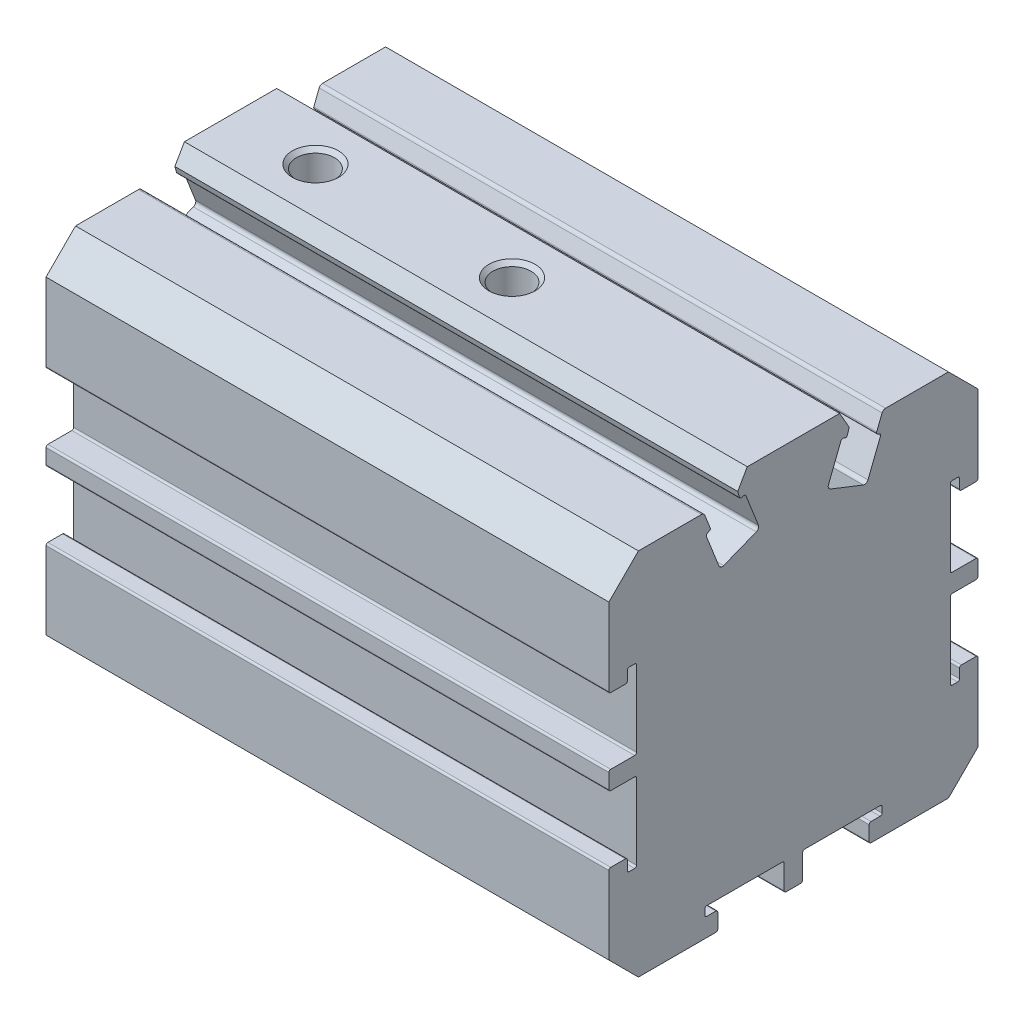
from build123d import *

# Parameters (mm, degrees)
BOSS_EXTRUDE1_DEPTH  = 61
LPATTERN1_COUNT      = 2
LPATTERN1_PITCH      = 28
LPATTERN1_COUNT_DIR2 = 2
LPATTERN1_PITCH_DIR2 = 28
BOSS_EXTRUDE2_START  = 1.2
SKETCH8_R            = 1
BOSS_EXTRUDE2_DEPTH  = 1.2


with BuildPart() as part:
    # Sketch1 → Boss-Extrude1 (new body)
    with BuildSketch(Plane(origin=(0, 0, 0), x_dir=(0, 0, -1), z_dir=(1, 0, 0))):
        with BuildLine():
            Line((-20, 16.8), (-20, 8.4))
            ThreePointArc((-20, 8.4), (-19.941421356, 8.258578644), (-19.8, 8.2))
            Line((-19.8, 8.2), (-18.2, 8.2))
            ThreePointArc((-18.2, 8.2), (-18.058578644, 8.258578644), (-18, 8.4))
            Line((-18, 8.4), (-18, 9.4))
            ThreePointArc((-18, 9.4), (-17.941421356, 9.541421356), (-17.8, 9.6))
            Line((-17.8, 9.6), (-17.2, 9.6))
            ThreePointArc((-17.2, 9.6), (-17.058578644, 9.541421356), (-17, 9.4))
            Line((-17, 9.4), (-17, 1.2))
            ThreePointArc((-17, 1.2), (-17.058578644, 1.058578644), (-17.2, 1))
            Line((-17.2, 1), (-19.8, 1))
            ThreePointArc((-19.8, 1), (-19.941421356, 0.941421356), (-20, 0.8))
            Line((-20, 0.8), (-20, -0.8))
            ThreePointArc((-20, -0.8), (-19.941421356, -0.941421356), (-19.8, -1))
            Line((-19.8, -1), (-17.2, -1))
            ThreePointArc((-17.2, -1), (-17.058578644, -1.058578644), (-17, -1.2))
            Line((-17, -1.2), (-17, -9.4))
            ThreePointArc((-17, -9.4), (-17.058578644, -9.541421356), (-17.2, -9.6))
            Line((-17.2, -9.6), (-17.8, -9.6))
            ThreePointArc((-17.8, -9.6), (-17.941421356, -9.541421356), (-18, -9.4))
            Line((-18, -9.4), (-18, -8.4))
            ThreePointArc((-18, -8.4), (-18.058578644, -8.258578644), (-18.2, -8.2))
            Line((-18.2, -8.2), (-19.8, -8.2))
            ThreePointArc((-19.8, -8.2), (-19.941421356, -8.258578644), (-20, -8.4))
            Line((-20, -8.4), (-20, -16.8))
            Line((-20, -16.8), (-16.8, -20))
            Line((-16.8, -20), (-8.4, -20))
            ThreePointArc((-8.4, -20), (-8.258578644, -19.941421356), (-8.2, -19.8))
            Line((-8.2, -19.8), (-8.2, -18.2))
            ThreePointArc((-8.2, -18.2), (-8.258578644, -18.058578644), (-8.4, -18))
            Line((-8.4, -18), (-9.4, -18))
            ThreePointArc((-9.4, -18), (-9.541421356, -17.941421356), (-9.6, -17.8))
            Line((-9.6, -17.8), (-9.6, -17.2))
            ThreePointArc((-9.6, -17.2), (-9.541421356, -17.058578644), (-9.4, -17))
            Line((-9.4, -17), (-1.2, -17))
            ThreePointArc((-1.2, -17), (-1.058578644, -17.058578644), (-1, -17.2))
            Line((-1, -17.2), (-1, -19.8))
            ThreePointArc((-1, -19.8), (-0.941421356, -19.941421356), (-0.8, -20))
            Line((-0.8, -20), (0.8, -20))
            ThreePointArc((0.8, -20), (0.941421356, -19.941421356), (1, -19.8))
            Line((1, -19.8), (1, -17.2))
            ThreePointArc((1, -17.2), (1.058578644, -17.058578644), (1.2, -17))
            Line((1.2, -17), (9.4, -17))
            ThreePointArc((9.4, -17), (9.541421356, -17.058578644), (9.6, -17.2))
            Line((9.6, -17.2), (9.6, -17.8))
            ThreePointArc((9.6, -17.8), (9.541421356, -17.941421356), (9.4, -18))
            Line((9.4, -18), (8.4, -18))
            ThreePointArc((8.4, -18), (8.258578644, -18.058578644), (8.2, -18.2))
            Line((8.2, -18.2), (8.2, -19.8))
            ThreePointArc((8.2, -19.8), (8.258578644, -19.941421356), (8.4, -20))
            Line((8.4, -20), (16.8, -20))
            Line((16.8, -20), (20, -16.8))
            Line((20, -16.8), (20, -8.4))
            ThreePointArc((20, -8.4), (19.941421356, -8.258578644), (19.8, -8.2))
            Line((19.8, -8.2), (18.2, -8.2))
            ThreePointArc((18.2, -8.2), (18.058578644, -8.258578644), (18, -8.4))
            Line((18, -8.4), (18, -9.4))
            ThreePointArc((18, -9.4), (17.941421356, -9.541421356), (17.8, -9.6))
            Line((17.8, -9.6), (17.2, -9.6))
            ThreePointArc((17.2, -9.6), (17.058578644, -9.541421356), (17, -9.4))
            Line((17, -9.4), (17, -1.2))
            ThreePointArc((17, -1.2), (17.058578644, -1.058578644), (17.2, -1))
            Line((17.2, -1), (19.8, -1))
            ThreePointArc((19.8, -1), (19.941421356, -0.941421356), (20, -0.8))
            Line((20, -0.8), (20, 0.8))
            ThreePointArc((20, 0.8), (19.941421356, 0.941421356), (19.8, 1))
            Line((19.8, 1), (17.2, 1))
            ThreePointArc((17.2, 1), (17.058578644, 1.058578644), (17, 1.2))
            Line((17, 1.2), (17, 9.4))
            ThreePointArc((17, 9.4), (17.058578644, 9.541421356), (17.2, 9.6))
            Line((17.2, 9.6), (17.8, 9.6))
            ThreePointArc((17.8, 9.6), (17.941421356, 9.541421356), (18, 9.4))
            Line((18, 9.4), (18, 8.4))
            ThreePointArc((18, 8.4), (18.058578644, 8.258578644), (18.2, 8.2))
            Line((18.2, 8.2), (19.8, 8.2))
            ThreePointArc((19.8, 8.2), (19.941421356, 8.258578644), (20, 8.4))
            Line((20, 8.4), (20, 16.8))
            Line((20, 16.8), (16.8, 20))
            Line((16.8, 20), (9.977696427, 20))
            ThreePointArc((9.977696427, 20), (9.752574456, 19.9306359), (9.6055294, 19.746600491))
            Line((9.6055294, 19.746600491), (9.021684768, 18.264424545))
            ThreePointArc((9.021684768, 18.264424545), (9.024356267, 18.111374485), (9.134468036, 18.005040786))
            Line((9.134468036, 18.005040786), (9.32055155, 17.93174054))
            ThreePointArc((9.32055155, 17.93174054), (9.430663319, 17.825406841), (9.433334818, 17.672356781))
            Line((9.433334818, 17.672356781), (8.077280279, 14.22981178))
            ThreePointArc((8.077280279, 14.22981178), (7.86461288, 14.009588241), (7.558512761, 14.004245243))
            Line((7.558512761, 14.004245243), (4.022926003, 15.396949905))
            ThreePointArc((4.022926003, 15.396949905), (3.802702464, 15.609617305), (3.797359467, 15.915717423))
            Line((3.797359467, 15.915717423), (5.153414005, 19.358262424))
            ThreePointArc((5.153414005, 19.358262424), (5.259747705, 19.468374194), (5.412797764, 19.471045693))
            Line((5.412797764, 19.471045693), (5.580796856, 19.40486909))
            ThreePointArc((5.580796856, 19.40486909), (5.742251705, 19.411428885), (5.846162096, 19.535175925))
            Line((5.846162096, 19.535175925), (6.039230485, 20.2))
            Line((6.039230485, 20.2), (5, 22))
            Line((5, 22), (-5, 22))
            Line((-5, 22), (-6.039230485, 20.2))
            Line((-6.039230485, 20.2), (-5.846162096, 19.535175925))
            ThreePointArc((-5.846162096, 19.535175925), (-5.742251705, 19.411428885), (-5.580796856, 19.40486909))
            Line((-5.580796856, 19.40486909), (-5.412797764, 19.471045693))
            ThreePointArc((-5.412797764, 19.471045693), (-5.259747705, 19.468374194), (-5.153414005, 19.358262424))
            Line((-5.153414005, 19.358262424), (-3.797359467, 15.915717423))
            ThreePointArc((-3.797359467, 15.915717423), (-3.802702464, 15.609617305), (-4.022926003, 15.396949905))
            Line((-4.022926003, 15.396949905), (-7.558512761, 14.004245243))
            ThreePointArc((-7.558512761, 14.004245243), (-7.86461288, 14.009588241), (-8.077280279, 14.22981178))
            Line((-8.077280279, 14.22981178), (-9.433334818, 17.672356781))
            ThreePointArc((-9.433334818, 17.672356781), (-9.430663319, 17.825406841), (-9.32055155, 17.93174054))
            Line((-9.32055155, 17.93174054), (-9.134468036, 18.005040786))
            ThreePointArc((-9.134468036, 18.005040786), (-9.024356267, 18.111374485), (-9.021684768, 18.264424545))
            Line((-9.021684768, 18.264424545), (-9.6055294, 19.746600491))
            ThreePointArc((-9.6055294, 19.746600491), (-9.752574456, 19.9306359), (-9.977696427, 20))
            Line((-9.977696427, 20), (-16.8, 20))
            Line((-16.8, 20), (-20, 16.8))
        make_face()
    extrude(amount=BOSS_EXTRUDE1_DEPTH)

    # Sketch2 → Cut-Revolve1 (revolve, cut)
    with BuildSketch(Plane.XY.offset(14), mode=Mode.PRIVATE) as cut_revolve1_sk:
        Polygon((0, -14), (0, -9.65), (0.25, -9.9), (5.5, -9.9), (5.5, -11), (6.0415, -11.5415), (29.9585, -11.5415), (30.5, -11), (30.5, -9.9), (35.75, -9.9), (36, -9.65), (36, -14), align=None)
    cut_revolve1 = revolve(cut_revolve1_sk.sketch.rotate(Axis((36, -14, 14), (-1, 0, 0)), 270), axis=Axis((36, -14, 14), (-1, 0, 0)), mode=Mode.SUBTRACT)

    # LPattern1: Cut-Revolve1 2 × 2
    with Locations(*[(0, j * LPATTERN1_PITCH_DIR2, -i * LPATTERN1_PITCH) for i in range(LPATTERN1_COUNT) for j in range(LPATTERN1_COUNT_DIR2) if (i, j) != (0, 0)]):
        add(cut_revolve1, mode=Mode.SUBTRACT)

    # Sketch4 → Cut-Revolve2 (revolve, cut)
    with BuildSketch(Plane.XY, mode=Mode.PRIVATE) as cut_revolve2_sk:
        Polygon((9.2, 22), (11.7, 22), (11.267, 21.567), (11.267, 17), (9.2, 17), align=None)
    revolve(cut_revolve2_sk.sketch.rotate(Axis((9.2, 17, 0), (0, 1, 0)), 270), axis=Axis((9.2, 17, 0), (0, 1, 0)), mode=Mode.SUBTRACT)

    # Sketch5 → Cut-Revolve3 (revolve, cut)
    with BuildSketch(Plane.XY, mode=Mode.PRIVATE) as cut_revolve3_sk:
        Polygon((30.5, 22), (33, 22), (32.567, 21.567), (32.567, 17), (30.5, 17), align=None)
    revolve(cut_revolve3_sk.sketch.rotate(Axis((30.5, 17, 0), (0, 1, 0)), 270), axis=Axis((30.5, 17, 0), (0, 1, 0)), mode=Mode.SUBTRACT)

    # Sketch6 → Cut-Revolve4 (revolve, cut)
    with BuildSketch(Plane.XY, mode=Mode.PRIVATE) as cut_revolve4_sk:
        Polygon((0, 0), (0, 5), (10, 5), (10, 12.5), (57, 12.5), (57, 0), align=None)
    revolve(cut_revolve4_sk.sketch.rotate(Axis((57, 0, 0), (-1, 0, 0)), 270), axis=Axis((57, 0, 0), (-1, 0, 0)), mode=Mode.SUBTRACT)

    # Sketch7 → Cut-Revolve5 (revolve, cut)
    with BuildSketch(Plane.XY, mode=Mode.PRIVATE) as cut_revolve5_sk:
        Polygon((0, 0), (0, 14.3), (0.3, 14), (2.8, 14), (2.8, 0), align=None)
    revolve(cut_revolve5_sk.sketch.rotate(Axis((2.8, 0, 0), (-1, 0, 0)), 270), axis=Axis((2.8, 0, 0), (-1, 0, 0)), mode=Mode.SUBTRACT)

    # Sketch8 → Boss-Extrude2 (add)
    with BuildSketch(Plane(origin=(1.6, 0, 0), x_dir=(0, 0, -1), z_dir=(1, 0, 0)).offset(BOSS_EXTRUDE2_START)):
        with BuildLine():
            ThreePointArc((8.749790987, -10.928913839), (0, 14), (-8.749790987, -10.928913839))
            ThreePointArc((-8.749790987, -10.928913839), (-4.890371671, -11.636058747), (-8.188276559, -9.510266018))
            ThreePointArc((-8.188276559, -9.510266018), (-8.931435091, -9.815110466), (-9.659095382, -9.474926336))
            ThreePointArc((-9.659095382, -9.474926336), (0, 11.85), (9.659095382, -9.474926336))
            ThreePointArc((9.659095382, -9.474926336), (8.931435083, -9.815110467), (8.188276548, -9.510266007))
            ThreePointArc((8.188276548, -9.510266007), (4.890371674, -11.636058754), (8.749790987, -10.928913839))
        make_face()
        with Locations(Location((6.75, -10.9, 0), (0, 0, 180))):
            Circle(SKETCH8_R, mode=Mode.SUBTRACT)
        with Locations(Location((-6.75, -10.9, 0), (0, 0, 180))):
            Circle(SKETCH8_R, mode=Mode.SUBTRACT)
    extrude(amount=-BOSS_EXTRUDE2_DEPTH)

    # Sketch9 → Revolve1 (revolve)
    with BuildSketch(Plane.XY, mode=Mode.PRIVATE) as revolve1_sk:
        with BuildLine():
            Line((-2, 7.5), (-2, 5))
            Line((-2, 5), (2.8, 5))
            Line((2.8, 5), (2.8, 8.5))
            Line((2.8, 8.5), (-1, 8.5))
            ThreePointArc((-1, 8.5), (-1.707106781, 8.207106781), (-2, 7.5))
        make_face()
    revolve(revolve1_sk.sketch.rotate(Axis((2.8, 0, 0), (-1, 0, 0)), 270), axis=Axis((2.8, 0, 0), (-1, 0, 0)))

    # Sketch10 → Cut-Revolve6 (revolve, cut)
    with BuildSketch(Plane.XY, mode=Mode.PRIVATE) as cut_revolve6_sk:
        Polygon((58.5, 0), (58.5, 12.5), (59.75, 12.5), (60, 12.75), (60, 0), align=None)
    revolve(cut_revolve6_sk.sketch.rotate(Axis((60, 0, 0), (-1, 0, 0)), 180), axis=Axis((60, 0, 0), (-1, 0, 0)), mode=Mode.SUBTRACT)


solid = part.part
